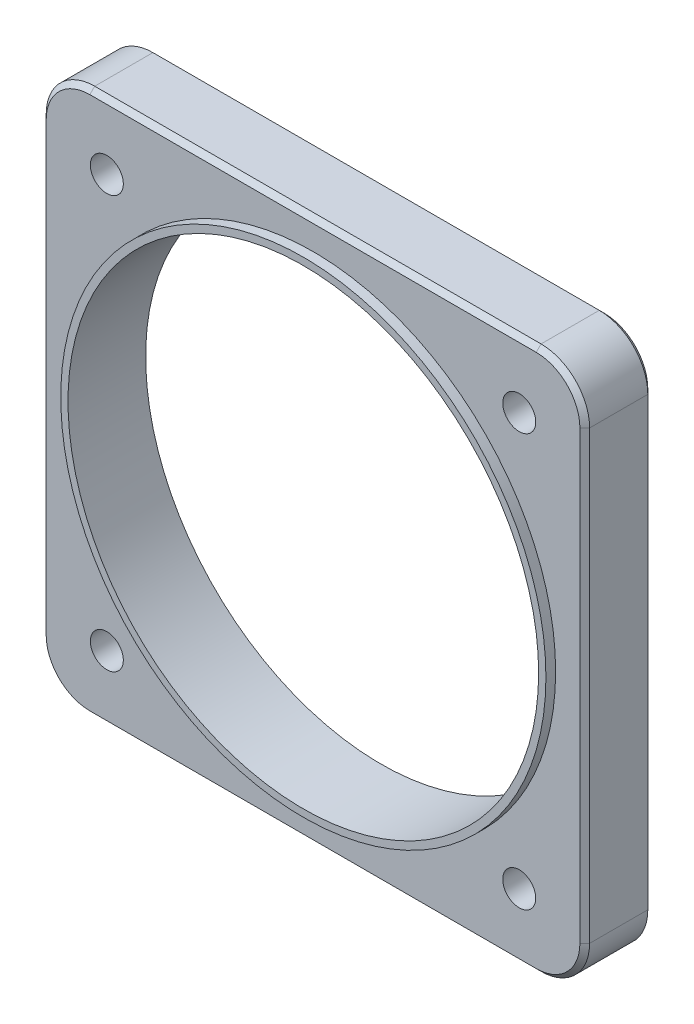
SolidWorks part; units mm, degrees
material "Q235B"
ref_plane "Front Plane" through (0, 0, 0) normal (0, 0, 1) x (1, 0, 0)
ref_plane "Top Plane" through (0, 0, 0) normal (0, 1, 0) x (1, 0, 0)
ref_plane "Right Plane" through (0, 0, 0) normal (1, 0, 0) x (0, 0, -1)
sketch "Sketch1" plane through (0, 0, 0) normal (0, 0, 1) x (1, 0, 0)
  line L1 (-46, 56) -> (46, 56)
  line L2 (-56, 46) -> (-56, -46)
  line L3 (-46, -56) -> (46, -56)
  line L4 (56, 46) -> (56, -46)
  line L5 (-56, 56) -> (56, -56) construction
  line L6 (-56, -56) -> (56, 56) construction
  arc A0 (-56, -46) -> (-46, -56) centre (-46, -46) ccw
  arc A1 (46, -56) -> (56, -46) centre (46, -46) ccw
  arc A2 (46, 56) -> (56, 46) centre (46, 46) cw
  arc A3 (-46, 56) -> (-56, 46) centre (-46, 46) ccw
  circle A4 centre (0, 0) radius 48.5
  point P0 (0, 0)
  dimension "D2" = 10
  dimension "D3" = 97
  dimension "D1" = 112
extrude "Boss-Extrude1" add sketch "Sketch1" along normal blind 16
sketch "Sketch2" plane through (0, 0, 16) normal (0, 0, 1) x (1, 0, 0)
  line L1 (-42.5, 42.5) -> (42.5, 42.5) construction
  line L2 (-42.5, 42.5) -> (-42.5, -42.5) construction
  line L3 (-42.5, -42.5) -> (42.5, -42.5) construction
  line L4 (42.5, 42.5) -> (42.5, -42.5) construction
  line L5 (-42.5, 42.5) -> (42.5, -42.5) construction
  line L6 (-42.5, -42.5) -> (42.5, 42.5) construction
  circle A0 centre (-42.5, 42.5) radius 3.35
  circle A1 centre (42.5, 42.5) radius 3.35
  circle A2 centre (42.5, -42.5) radius 3.35
  circle A3 centre (-42.5, -42.5) radius 3.35
  point P0 (0, 0)
  dimension "D2" = 6.7
  dimension "D1" = 85
extrude "Cut-Extrude1" cut sketch "Sketch2" against normal through all
hole_wizard "M8 Tapped Hole2" positions "Sketch3" profile "Sketch4" tap size "M8" standard "GB" end condition through all
sketch "Sketch3" plane through (0, 0, 16) normal (0, 0, 1) x (1, 0, 0)
  point P0 (-42.5, 42.5)
  point P3 (42.5, 42.5)
  point P6 (42.5, -42.5)
  point P9 (-42.5, -42.5)
sketch "Sketch4" plane through (-42.5, 42.5, 16) normal (1, 0, 0) x (0, -1, 0)
  line L0 (0, 0) -> (0, 16)
  line L1 (0, 16) -> (3.4, 16)
  line L2 (3.4, 16) -> (3.4, 0)
  line L5 (3.4, 0) -> (0, 0)
  line L11 (0, -6.35) -> (0, 107.95) construction
  dimension "通孔螺纹孔钻头直径" = 6.8
  dimension "通孔螺纹孔钻头深度" = 16
cosmetic thread "Hole cosmetic thread1" parameters "D2"=8
cosmetic thread "Hole cosmetic thread2" parameters "D2"=8
cosmetic thread "Hole cosmetic thread3" parameters "D2"=8
cosmetic thread "Hole cosmetic thread4" parameters "D2"=8
sketch "Sketch5" plane through (0, 0, 16) normal (0, 0, 1) x (1, 0, 0)
  line L0 (56, -46) -> (56, 46) construction
  line L1 (-46, -56) -> (46, -56) construction
  line L2 (-56, 46) -> (-56, -46) construction
  line L3 (46, 56) -> (-46, 56) construction
  line L4 (56, -46) -> (56, 46)
  line L5 (-46, -56) -> (46, -56)
  line L6 (-56, 46) -> (-56, -46)
  line L7 (46, 56) -> (-46, 56)
  circle A0 centre (0, 0) radius 50
  arc A1 (56, 46) -> (46, 56) centre (46, 46) ccw construction
  arc A2 (46, -56) -> (56, -46) centre (46, -46) ccw construction
  arc A3 (-56, -46) -> (-46, -56) centre (-46, -46) ccw construction
  arc A4 (-46, 56) -> (-56, 46) centre (-46, 46) ccw construction
  arc A5 (56, 46) -> (46, 56) centre (46, 46) ccw
  arc A6 (46, -56) -> (56, -46) centre (46, -46) ccw
  arc A7 (-56, -46) -> (-46, -56) centre (-46, -46) ccw
  arc A8 (-46, 56) -> (-56, 46) centre (-46, 46) ccw
  dimension "D1" = 100
extrude "Cut-Extrude2" cut sketch "Sketch5" against normal blind 2
chamfer "Chamfer1" distance 1 angle 45 16 edges at (56, 0, 14) (53.0711, 53.0711, 14) (53.0711, -53.0711, 14) (0, 56, 14) (0, -56, 14) (-53.0711, 53.0711, 14) (-53.0711, -53.0711, 14) (-56, 0, 14) (56, 0, 0) (53.0711, 53.0711, 0) (53.0711, -53.0711, 0) (0, 56, 0) (0, -56, 0) (-53.0711, 53.0711, 0) (-53.0711, -53.0711, 0) (-56, 0, 0)
